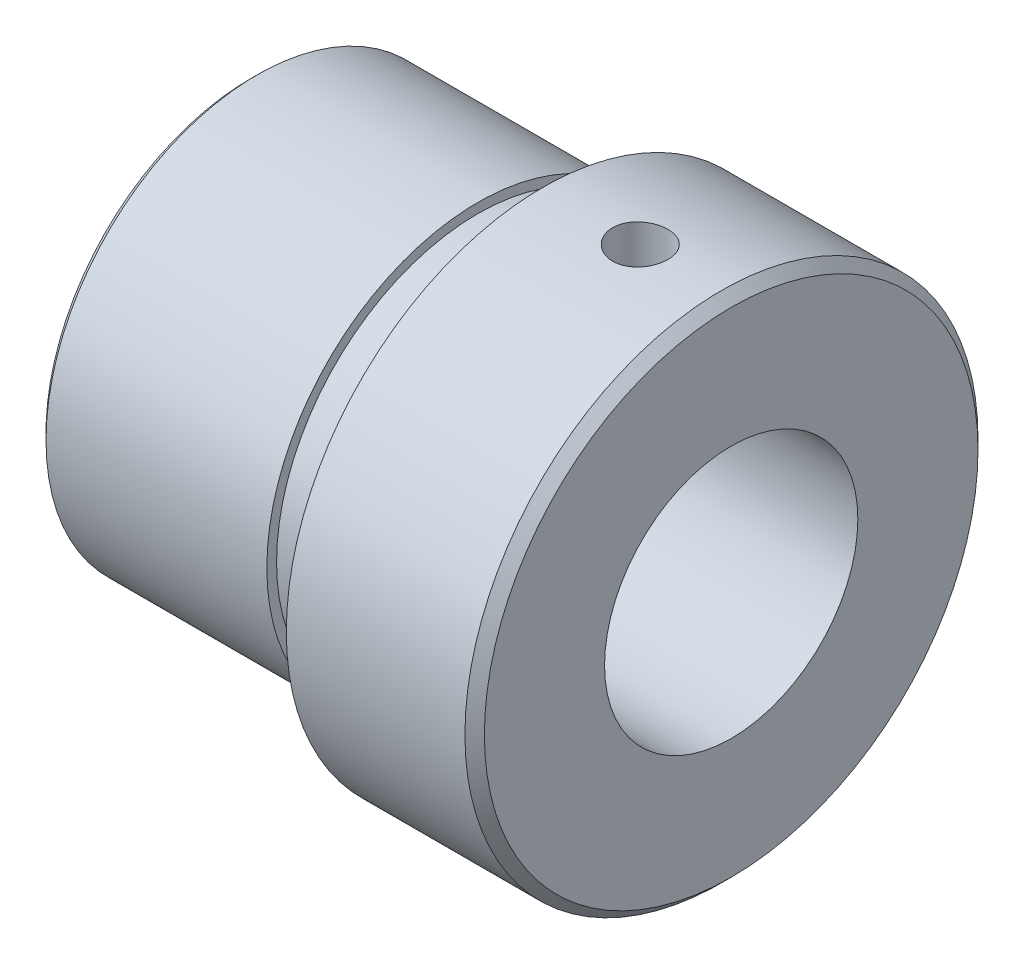
SolidWorks part; units mm, degrees
material "普通碳钢"
ref_plane "Front Plane" through (0, 0, 0) normal (0, 0, 1) x (1, 0, 0)
ref_plane "Top Plane" through (0, 0, 0) normal (0, 1, 0) x (1, 0, 0)
ref_plane "Right Plane" through (0, 0, 0) normal (1, 0, 0) x (0, 0, -1)
sketch "Sketch1" plane through (0, 0, 0) normal (1, 0, 0) x (0, 0, -1)
  circle A0 centre (0, 0) radius 39.5
  dimension "D1" = 79
extrude "Boss-Extrude1" add sketch "Sketch1" along normal blind 144
sketch "Sketch2" plane through (144, 0, 0) normal (1, 0, 0) x (0, 0, -1)
  circle A0 centre (0, 0) radius 22.5
  dimension "D1" = 45
extrude "Cut-Extrude1" cut sketch "Sketch2" against normal blind 70 flip side to cut
cosmetic thread "Cosmetic Thread2" parameters "D2"=31
sketch "Sketch4" plane through (0, 0, 0) normal (-1, 0, 0) x (0, 0, 1)
  circle A0 centre (0, 0) radius 32.5
  dimension "D1" = 65
extrude "Cut-Extrude3" cut sketch "Sketch4" against normal blind 45 flip side to cut
cosmetic thread "Cosmetic Thread3" parameters "D2"=63.5
sketch "Sketch5" plane through (74, 0, 0) normal (1, 0, 0) x (0, 0, -1)
  circle A0 centre (0, 0) radius 16.75
  dimension "D1" = 33.5
extrude "Cut-Extrude4" [suppressed] cut sketch "Sketch5" along normal blind 2.5 flip side to cut
sketch "Sketch6" plane through (45, 0, 0) normal (-1, 0, 0) x (0, 0, 1)
  circle A0 centre (0, 0) radius 31
  dimension "D1" = 62
extrude "Cut-Extrude5" cut sketch "Sketch6" along normal blind 10 flip side to cut
sketch "Sketch7" plane through (0, 0, 0) normal (0, 1, 0) x (1, 0, 0)
  line L0 (0, 0) -> (103.4655, 0) construction
  line L1 (48.5, 49.1063) -> (86.6903, 49.1063)
  line L2 (48.5, 49.1063) -> (48.5, 35)
  line L3 (48.5, 35) -> (86.6903, 35)
  line L4 (86.6903, 49.1063) -> (86.6903, 35)
  line L5 (48.5, 49.1063) -> (86.6903, 35) construction
  line L6 (48.5, 35) -> (86.6903, 49.1063) construction
  line L7 (48.5, -35) -> (100.0884, -35)
  line L8 (48.5, -35) -> (48.5, -45.5691)
  line L9 (48.5, -45.5691) -> (100.0884, -45.5691)
  line L10 (100.0884, -35) -> (100.0884, -45.5691)
  line L11 (48.5, -35) -> (100.0884, -45.5691) construction
  line L12 (48.5, -45.5691) -> (100.0884, -35) construction
  line L13 (74, -39.5) -> (74, 39.5) construction
  point P0 (67.5952, 42.0532)
  point P5 (74.2942, -40.2846)
  point P14 (74.2942, -35)
  dimension "D1" = 70
  dimension "D2" = 25.5
extrude "Cut-Extrude6" [suppressed] cut sketch "Sketch7" against normal through all both and the other way through all
draft "Draft2" [suppressed] type of draft neutral plane draft angle 45 faces to draft 1 parameters "D1"=45
draft "Draft3" [suppressed] type of draft neutral plane draft angle 45 faces to draft 1 parameters "D1"=45
chamfer "Chamfer1" distance 1 angle 45 2 edges at (144, 0, -22.5) (0, 0, 32.5)
other "Move Face1" [suppressed] parameters "D1"=35
chamfer "Chamfer2" [suppressed] distance 1 angle 45
chamfer "Chamfer3" [suppressed] distance 1 angle 45
sketch "Sketch8" plane through (74, 0, 0) normal (1, 0, 0) x (0, 0, -1)
  line L0 (-52.7946, 0) -> (49.241, 0) construction
  line L1 (0, 35) -> (-30.3109, 17.5)
  line L2 (-30.3109, 17.5) -> (-30.3109, -17.5)
  line L3 (-30.3109, -17.5) -> (0, -35)
  line L4 (0, -35) -> (30.3109, -17.5)
  line L5 (30.3109, -17.5) -> (30.3109, 17.5)
  line L6 (30.3109, 17.5) -> (0, 35)
  circle A0 centre (0, 0) radius 35 construction
  dimension "D1" = 70
extrude "Cut-Extrude7" [suppressed] cut sketch "Sketch8" against normal blind 22 flip side to cut
fillet "Fillet1" [suppressed] radius 5
chamfer "Chamfer4" [suppressed] distance 5 angle 45
sketch "Sketch9" [suppressed] plane through (63, 0, 0) normal (1, 0, 0) x (0, 0, -1)
  circle A0 centre (0, 0) radius 35
  dimension "D1" = 70
extrude "Boss-Extrude2" [suppressed] add sketch "Sketch9" along normal blind 4.5
chamfer "Chamfer5" [suppressed] distance 4.5 angle 45
chamfer "Chamfer6" [suppressed] distance 0.3 angle 45
chamfer "Chamfer7" distance 1.5 angle 45 1 edges at (74, 0, -39.5)
ref_plane "Plane1" through (0, -39.5, 0) normal (0, -1, 0) x (-1, 0, 0)
sketch "Sketch12" plane through (0, -39.5, 0) normal (0, -1, 0) x (-1, 0, 0)
  line L0 (-45, -39.5) -> (-45, 39.5) construction
  circle A0 centre (-60, 0) radius 4.25
  dimension "D2" = 8.5
  dimension "D1" = 15
extrude "Cut-Extrude8" cut sketch "Sketch12" against normal blind 2
cosmetic thread "孔螺蚊线2" parameters "D1"=12, "D2"=10
hole_wizard "M10 Tapped Hole1" positions "Sketch13" profile "Sketch14" tap size "M10" standard "GB"
sketch "Sketch13" plane through (0, -37.5, 0) normal (0, -1, 0) x (-1, 0, 0)
  point P0 (-60, 0)
sketch "Sketch14" plane through (60, -37.5, 0) normal (1, 0, 0) x (0, 0, -1)
  line L0 (0, 0) -> (0, 12.5537)
  line L1 (0, 12.5537) -> (4.25, 10)
  line L2 (4.25, 10) -> (4.25, 0)
  line L5 (4.25, 0) -> (0, 0)
  line L10 (0, 12.5537) -> (-4.25, 10) construction
  line L11 (0, -6.35) -> (0, 107.95) construction
  dimension "螺纹孔钻头直径" = 8.5
  dimension "螺纹孔钻头深度" = 10
  dimension "导头角度" = 118
mirror "Mirror1" about plane through (0, 0, 0) normal (0, 1, 0) of "M10 Tapped Hole1", "Cut-Extrude8"
sketch "Sketch15" plane through (144, 0, 0) normal (1, 0, 0) x (0, 0, -1)
  circle A0 centre (0, 0) radius 63.7384
extrude "Cut-Extrude9" cut sketch "Sketch15" against normal up to surface (70 mm away) up to face at (74, 0, -38)
hole_wizard "M42x3.0 Tapped Hole1" positions "Sketch16" profile "Sketch17" tap size "M42x3.0" standard "GB" end condition through all
sketch "Sketch16" plane through (74, 0, 0) normal (1, 0, 0) x (0, 0, -1)
  point P0 (0, 0)
sketch "Sketch17" plane through (74, 0, 0) normal (0, 1, 0) x (0, 0, -1)
  line L0 (0, 0) -> (0, 74)
  line L1 (0, 74) -> (19.5, 74)
  line L2 (19.5, 74) -> (19.5, 0)
  line L5 (19.5, 0) -> (0, 0)
  line L11 (0, -6.35) -> (0, 107.95) construction
  dimension "通孔螺纹孔钻头直径" = 39
  dimension "通孔螺纹孔钻头深度" = 74
cosmetic thread "Cosmetic Thread1" parameters "D2"=42
